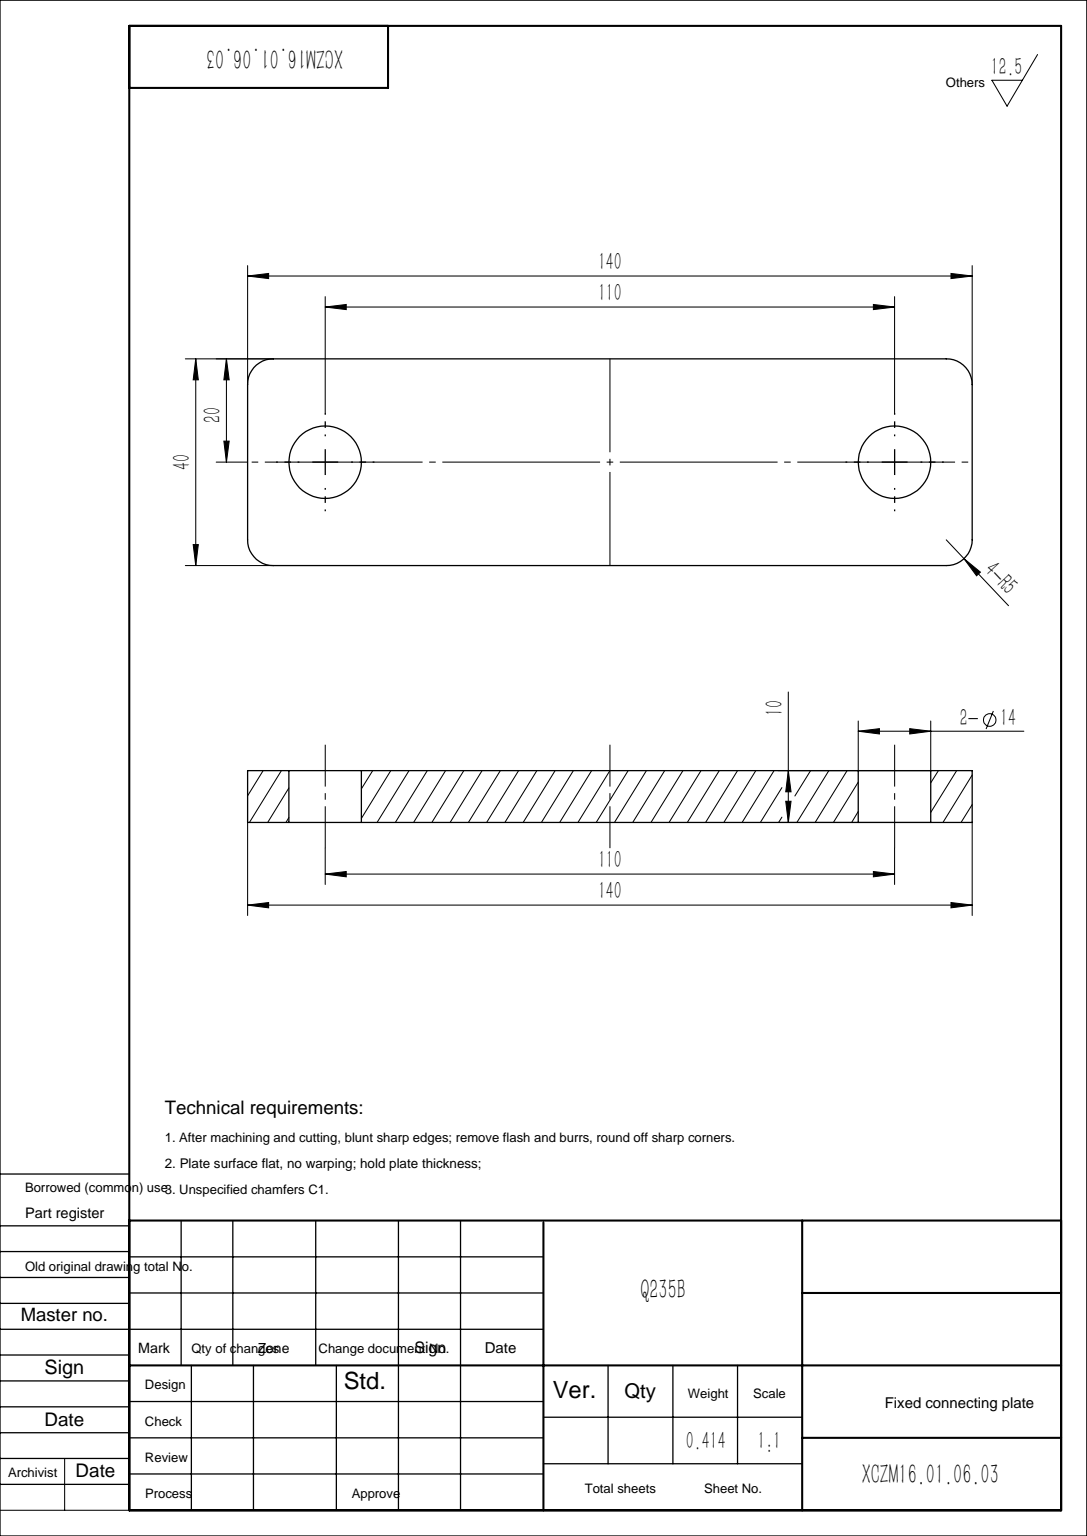
from build123d import *

# Parameters (mm, degrees)
SKETCH2_R           = 7
BOSS_EXTRUDE1_DEPTH = 10


with BuildPart() as part:
    # Sketch2 → Boss-Extrude1 (new body)
    with BuildSketch(Plane(origin=(0, 0, 0), x_dir=(1, 0, 0), z_dir=(0, 1, 0))):
        with BuildLine():
            Line((65, -20), (-65, -20))
            ThreePointArc((-65, -20), (-68.535533906, -18.535533906), (-70, -15))
            Line((-70, -15), (-70, 15))
            ThreePointArc((-70, 15), (-68.535533906, 18.535533906), (-65, 20))
            Line((-65, 20), (65, 20))
            ThreePointArc((65, 20), (68.535533906, 18.535533906), (70, 15))
            Line((70, 15), (70, -15))
            ThreePointArc((70, -15), (68.535533906, -18.535533906), (65, -20))
        make_face()
        with Locations(Location((-55, 0, 0), (0, 0, 270))):
            Circle(SKETCH2_R, mode=Mode.SUBTRACT)
        with Locations(Location((55, 0, 0), (0, 0, 90))):
            Circle(SKETCH2_R, mode=Mode.SUBTRACT)
    extrude(amount=BOSS_EXTRUDE1_DEPTH)


solid = part.part
